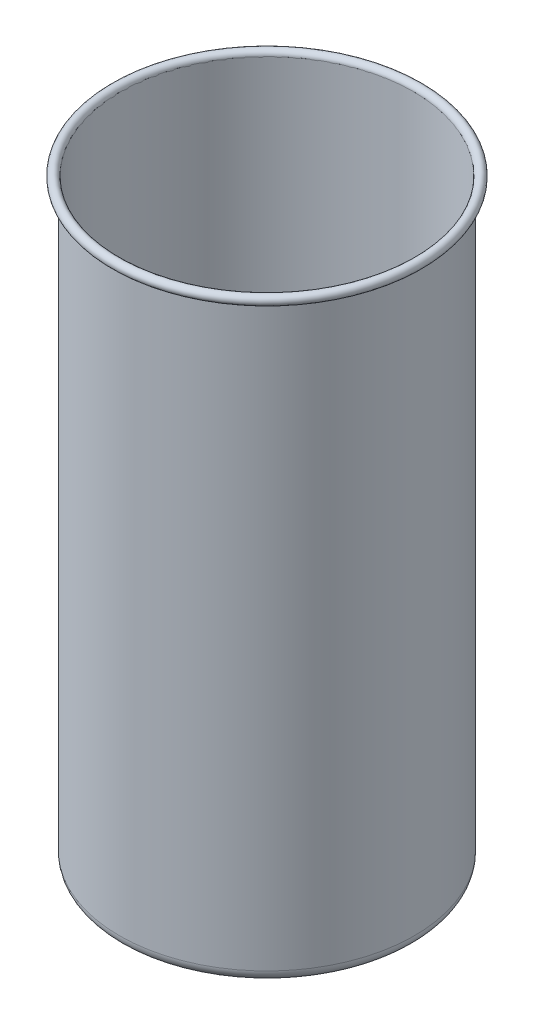
SolidWorks part; units mm, degrees
material "AISI 304"
ref_plane "Front Plane" through (0, 0, 0) normal (0, 0, 1) x (1, 0, 0)
ref_plane "Top Plane" through (0, 0, 0) normal (0, 1, 0) x (1, 0, 0)
ref_plane "Right Plane" through (0, 0, 0) normal (1, 0, 0) x (0, 0, -1)
sketch "Sketch1" plane through (0, 0, 0) normal (0, 1, 0) x (1, 0, 0)
  circle A0 centre (0, 0) radius 125
  dimension "D1" = 250
extrude "Boss-Extrude1" add sketch "Sketch1" along normal blind 505
fillet "Fillet1" radius 10 1 edges at (0, 0, 125)
shell "Shell1" thickness 1
sketch "Sketch6" plane through (0, 0, 0) normal (0, 0, 1) x (1, 0, 0)
  line L0 (125, 505) -> (-125, 505) construction
  line L1 (125, 505) -> (-125, 505) construction
  line L2 (125, 505) -> (125, 405) construction
  line L3 (125, 10) -> (125, 505) construction
  line L4 (125, 405) -> (-125, 405) construction
  line L5 (-125, 505) -> (-125, 10) construction
  line L6 (-125, 405) -> (-125, 505) construction
  line L7 (124, 505) -> (124, 405) construction
  line L8 (0, 505) -> (0, 726.7318) construction
  line L9 (128, 505) -> (124, 505) construction
  circle A1 centre (128, 505) radius 4
  circle A2 centre (128, 505) radius 3
  dimension "D2" = 8
  dimension "D3" = 1
  dimension "D1" = 100
  dimension "D4" = 1
revolve "Revolve1" add sketch "Sketch6" angle 360 about L8
